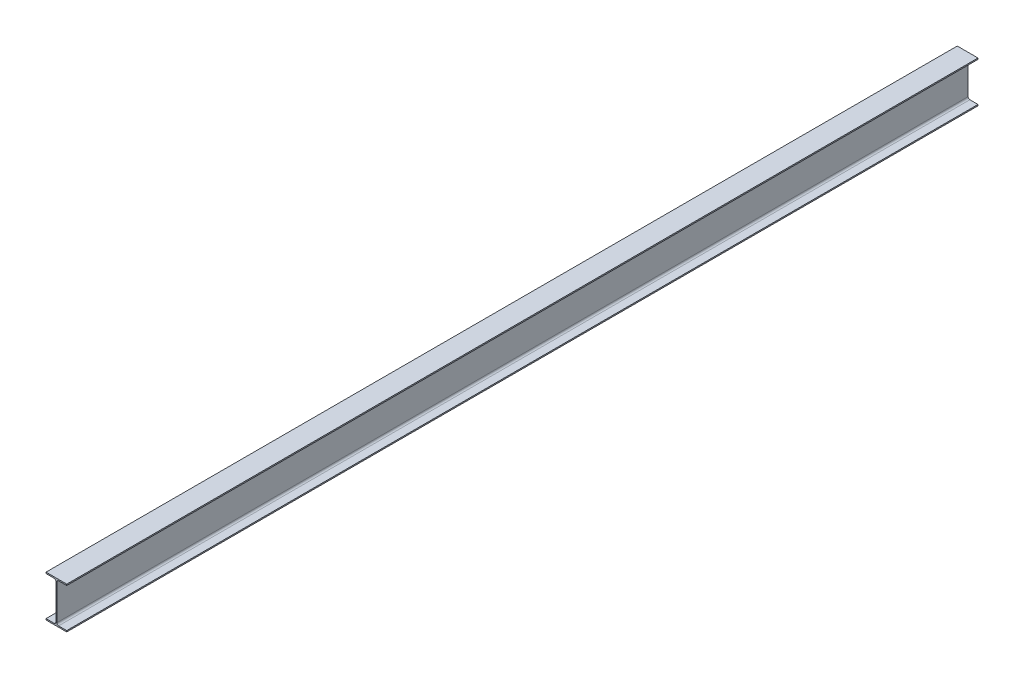
from build123d import *

# Parameters (mm, degrees)
BOSS_EXTRUDE1_DEPTH = 6592


with BuildPart() as part:
    # Sketch1 → Boss-Extrude1 (new body)
    with BuildSketch(Plane.XY):
        with BuildLine():
            Line((75, 0), (-75, 0))
            Line((-75, 0), (-75, 9))
            Line((-75, 9), (-16.25, 9))
            ThreePointArc((-16.25, 9), (-7.057611845, 12.807611845), (-3.25, 22))
            Line((-3.25, 22), (-3.25, 278))
            ThreePointArc((-3.25, 278), (-7.057611845, 287.192388155), (-16.25, 291))
            Line((-16.25, 291), (-75, 291))
            Line((-75, 291), (-75, 300))
            Line((-75, 300), (75, 300))
            Line((75, 300), (75, 291))
            Line((75, 291), (16.25, 291))
            ThreePointArc((16.25, 291), (7.057611845, 287.192388155), (3.25, 278))
            Line((3.25, 278), (3.25, 22))
            ThreePointArc((3.25, 22), (7.057611845, 12.807611845), (16.25, 9))
            Line((16.25, 9), (75, 9))
            Line((75, 9), (75, 0))
        make_face()
    extrude(amount=BOSS_EXTRUDE1_DEPTH)


solid = part.part
